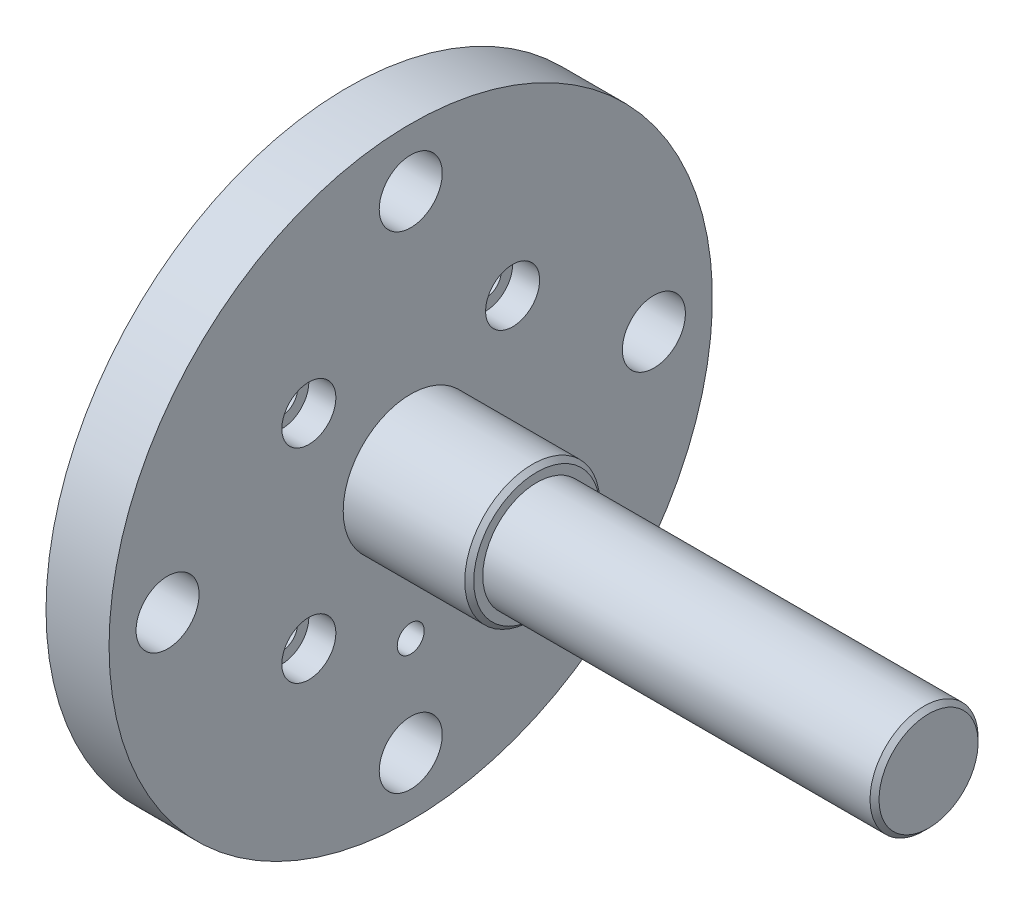
from build123d import *

# Parameters (mm, degrees)
SKETCH2_R           = 3.5
CUT_EXTRUDE1_DEPTH  = 27
SKETCH3_R           = 5.5
CUT_EXTRUDE2_DEPTH  = 6
CIRPATTERN1_COUNT   = 4
CHAMFER1_SIZE       = 1
SKETCH4_R           = 52.910606105
CUT_EXTRUDE3_DEPTH  = 128
SKETCH5_R           = 67
BOSS_EXTRUDE1_DEPTH = 14
SKETCH6_R           = 19
BOSS_EXTRUDE2_DEPTH = 5
SKETCH7_R           = 3
SKETCH7_R_2         = 3.5
CUT_EXTRUDE4_DEPTH  = 41
SKETCH8_R           = 6
CUT_EXTRUDE5_DEPTH  = 6
CHAMFER2_SIZE       = 1
SKETCH9_R           = 7
CUT_EXTRUDE6_DEPTH  = 41
CIRPATTERN2_COUNT   = 4


with BuildPart() as part:
    # Sketch1 → Revolve1 (revolve)
    with BuildSketch(Plane.XY, mode=Mode.PRIVATE) as revolve1_sk:
        Polygon((0, 0), (0, 8), (75, 8), (75, 17.5), (82, 17.5), (82, 34), (92, 34), (92, 15), (120, 15), (120, 12), (207, 12), (207, 0), align=None)
    revolve(revolve1_sk.sketch.rotate(Axis((0, 0, 0), (1, 0, 0)), 90), axis=Axis((0, 0, 0), (1, 0, 0)))

    # Sketch2 → Cut-Extrude1 (cut)
    with BuildSketch(Plane(origin=(92, 0, 0), x_dir=(0, 0, -1), z_dir=(1, 0, 0))):
        with Locations((0, 24.5)):
            Circle(SKETCH2_R)
    cut_extrude1 = extrude(amount=-CUT_EXTRUDE1_DEPTH, mode=Mode.SUBTRACT)

    # Sketch3 → Cut-Extrude2 (cut)
    with BuildSketch(Plane.ZY.offset(-82)):
        with Locations((0, 24.5)):
            Circle(SKETCH3_R)
    cut_extrude2 = extrude(amount=-CUT_EXTRUDE2_DEPTH, mode=Mode.SUBTRACT)

    # CirPattern1: Cut-Extrude1, Cut-Extrude2 ×4 about axis
    cirpattern1_axis = Axis((0, 0, 0), (1, 0, 0))
    add([cut_extrude1.rotate(cirpattern1_axis, i * 360 / CIRPATTERN1_COUNT) for i in range(1, CIRPATTERN1_COUNT)], mode=Mode.SUBTRACT)
    add([cut_extrude2.rotate(cirpattern1_axis, i * 360 / CIRPATTERN1_COUNT) for i in range(1, CIRPATTERN1_COUNT)], mode=Mode.SUBTRACT)

    # Chamfer1
    chamfer1_edges = [part.edges().sort_by_distance(p)[0] for p in [
        (82, 0, -34),
        (75, 0, -17.5),
        (75, 0, -8),
        (0, 0, -8),
        (207, 0, -12),
        (120, 0, -15),
    ]]
    chamfer(chamfer1_edges, length=CHAMFER1_SIZE)

    # Sketch4 → Cut-Extrude3 (cut)
    with BuildSketch(Plane(origin=(92, 0, 0), x_dir=(0, 0, -1), z_dir=(1, 0, 0))):
        Circle(SKETCH4_R)
    extrude(amount=-CUT_EXTRUDE3_DEPTH, mode=Mode.SUBTRACT)

    # Sketch5 → Boss-Extrude1 (add)
    with BuildSketch(Plane.ZY.offset(-92)):
        Circle(SKETCH5_R)
    extrude(amount=BOSS_EXTRUDE1_DEPTH)

    # Sketch6 → Boss-Extrude2 (add)
    with BuildSketch(Plane.ZY.offset(-78)):
        Circle(SKETCH6_R)
    extrude(amount=BOSS_EXTRUDE2_DEPTH)

    # Sketch7 → Cut-Extrude4 (cut)
    with BuildSketch(Plane.ZY.offset(-78)):
        with Locations((0, -32)):
            Circle(SKETCH7_R)
        with Locations((22.627416998, 22.627416998)):
            Circle(SKETCH7_R_2)
        with Locations((22.627416998, -22.627416998)):
            Circle(SKETCH7_R_2)
        with Locations((-22.627416998, -22.627416998)):
            Circle(SKETCH7_R_2)
        with Locations((-22.627416998, 22.627416998)):
            Circle(SKETCH7_R_2)
    extrude(amount=-CUT_EXTRUDE4_DEPTH, mode=Mode.SUBTRACT)

    # Sketch8 → Cut-Extrude5 (cut)
    with BuildSketch(Plane(origin=(92, 0, 0), x_dir=(0, 0, -1), z_dir=(1, 0, 0))):
        with Locations((22.627416998, 22.627416998)):
            Circle(SKETCH8_R)
        with Locations((22.627416998, -22.627416998)):
            Circle(SKETCH8_R)
        with Locations((-22.627416998, -22.627416998)):
            Circle(SKETCH8_R)
        with Locations((-22.627416998, 22.627416998)):
            Circle(SKETCH8_R)
    extrude(amount=-CUT_EXTRUDE5_DEPTH, mode=Mode.SUBTRACT)

    # Chamfer2
    chamfer2_edges = [part.edges().sort_by_distance(p)[0] for p in [
        (73, 0, -19),
    ]]
    chamfer(chamfer2_edges, length=CHAMFER2_SIZE)

    # Sketch9 → Cut-Extrude6 (cut)
    with BuildSketch(Plane.ZY.offset(-78)):
        with Locations((0, -54)):
            Circle(SKETCH9_R)
    cut_extrude6 = extrude(amount=-CUT_EXTRUDE6_DEPTH, mode=Mode.SUBTRACT)

    # CirPattern2: Cut-Extrude6 ×4 about axis
    cirpattern2_axis = Axis((0, 0, 0), (1, 0, 0))
    for i in range(1, CIRPATTERN2_COUNT):
        add(cut_extrude6.rotate(cirpattern2_axis, i * 360 / CIRPATTERN2_COUNT), mode=Mode.SUBTRACT)


solid = part.part
